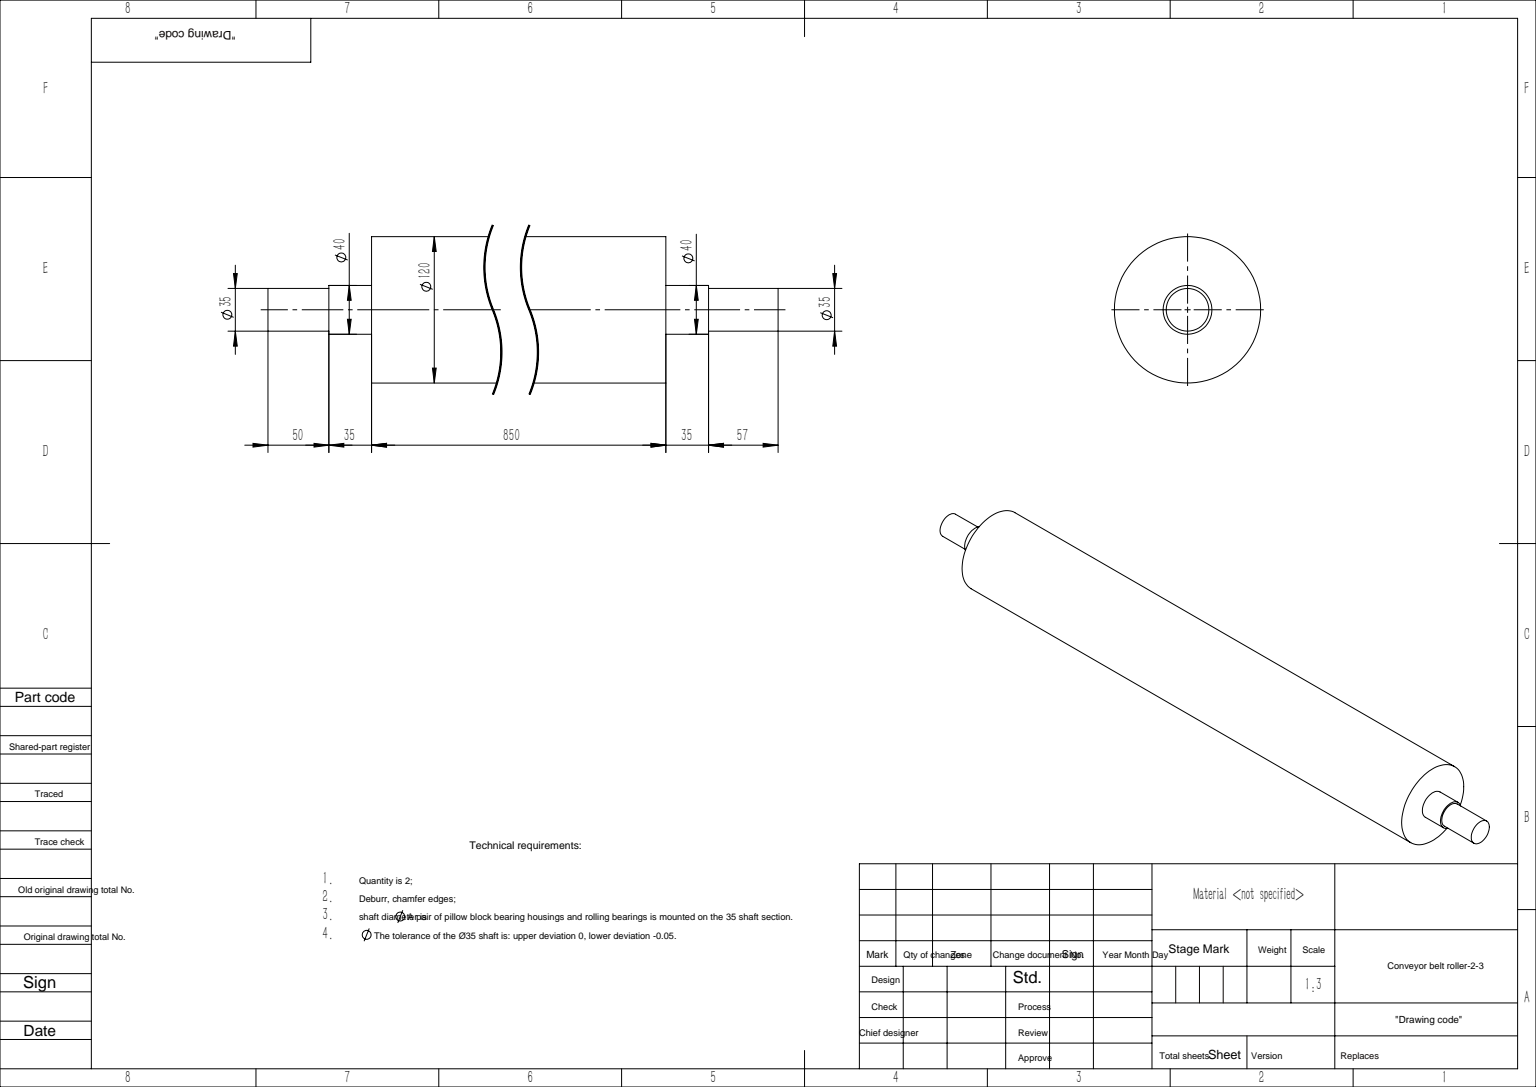
SolidWorks part; units mm, degrees
ref_plane "前视基准面" through (0, 0, 0) normal (0, 0, 1) x (1, 0, 0)
ref_plane "上视基准面" through (0, 0, 0) normal (0, 1, 0) x (1, 0, 0)
ref_plane "右视基准面" through (0, 0, 0) normal (1, 0, 0) x (0, 0, -1)
sketch "草图1" plane through (0, 0, 0) normal (0, 0, 1) x (1, 0, 0)
  line L0 (0, 0) -> (0, 17.5)
  line L1 (0, 17.5) -> (50, 17.5)
  line L2 (85, 20) -> (85, 60)
  line L3 (85, 60) -> (935, 60)
  line L4 (935, 60) -> (935, 20)
  line L5 (970, 17.5) -> (1027, 17.5)
  line L6 (1027, 17.5) -> (1027, 0)
  line L9 (1027, 0) -> (0, 0)
  line L10 (50, 17.5) -> (50, 20)
  line L11 (50, 20) -> (85, 20)
  line L12 (935, 20) -> (970, 20)
  line L13 (970, 20) -> (970, 17.5)
  dimension "D2" = 850
  dimension "D3" = 35
  dimension "D5" = 60
  dimension "D6" = 17.5
  dimension "D7" = 17.5
  dimension "D9" = 20
  dimension "D10" = 35
  dimension "D11" = 50
  dimension "D12" = 20
  dimension "D13" = 57
revolve "旋转1" add sketch "草图1" angle 360 about L9
